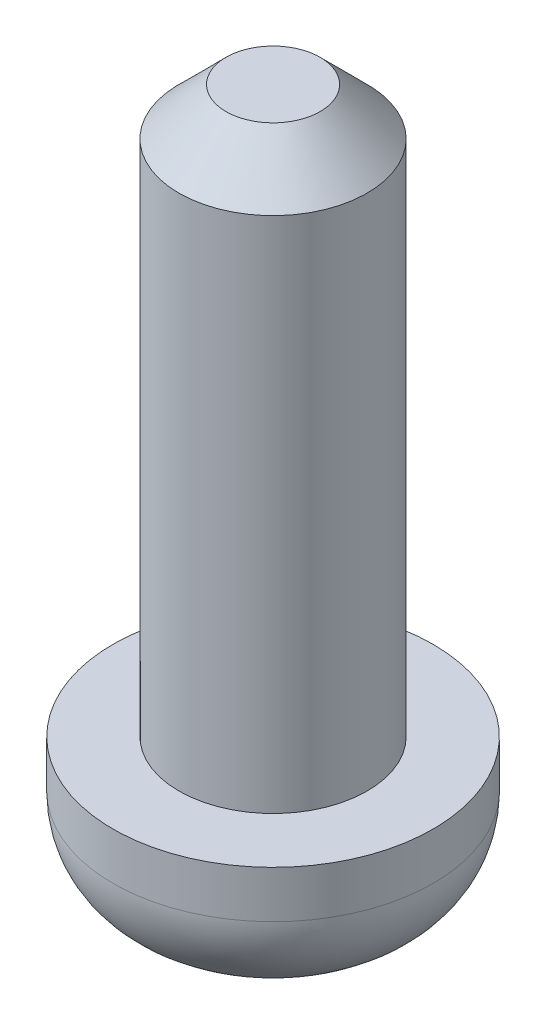
from build123d import *

# Parameters (mm, degrees)
SKETCH1_R           = 1
BOSS_EXTRUDE1_DEPTH = 6
CHAMFER1_SIZE       = 0.5
SKETCH2_R           = 1.7
BOSS_EXTRUDE2_DEPTH = 1.5
FILLET1_R           = 1


with BuildPart() as part:
    # Sketch1 → Boss-Extrude1 (new body)
    with BuildSketch(Plane(origin=(0, 0, 0), x_dir=(1, 0, 0), z_dir=(0, 1, 0))):
        with Locations(Location((0, 0, 0), (0, 0, 270))):
            Circle(SKETCH1_R)
    extrude(amount=BOSS_EXTRUDE1_DEPTH)

    # Chamfer1
    chamfer1_edges = [part.edges().sort_by_distance(p)[0] for p in [
        (0, 6, -1),
    ]]
    chamfer(chamfer1_edges, length=CHAMFER1_SIZE)

    # Sketch2 → Boss-Extrude2 (add)
    with BuildSketch(Plane.XZ):
        with Locations(Location((0, 0, 0), (0, 0, 270))):
            Circle(SKETCH2_R)
    extrude(amount=BOSS_EXTRUDE2_DEPTH)

    # Fillet1
    fillet1_edges = [part.edges().sort_by_distance(p)[0] for p in [
        (0, -1.5, 1.7),
    ]]
    fillet(fillet1_edges, radius=FILLET1_R)


solid = part.part
